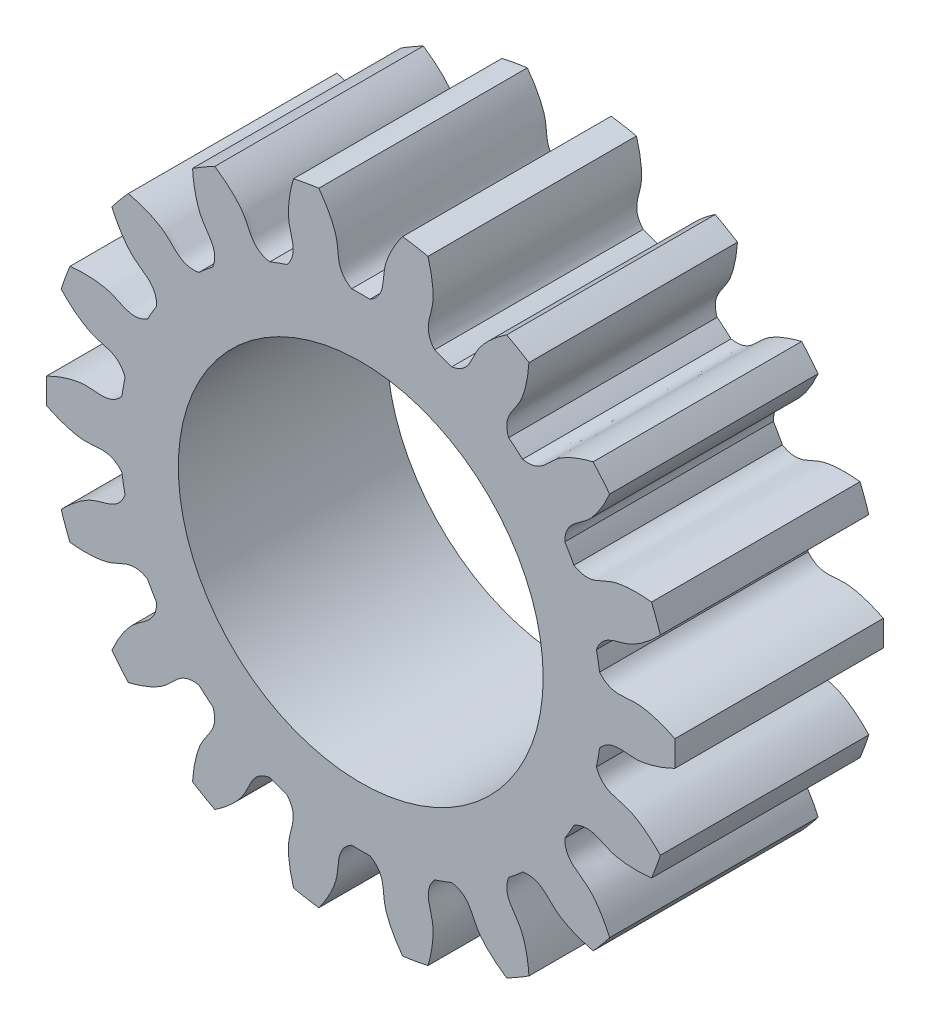
from build123d import *

# Parameters (mm, degrees)
SKETCH1_R           = 12.0625
BOSS_EXTRUDE1_DEPTH = 8
CUT_EXTRUDE1_DEPTH  = 19.841651002
CIRPATTERN1_COUNT   = 18
SKETCH4_R           = 7
CUT_EXTRUDE2_DEPTH  = 10


with BuildPart() as part:
    # Sketch1 → Boss-Extrude1 (new body)
    with BuildSketch(Plane.XY):
        Circle(SKETCH1_R)
    extrude(amount=BOSS_EXTRUDE1_DEPTH)

    # Sketch2 → Cut-Extrude1 (cut, through all)
    with BuildSketch(Plane.XY):
        with BuildLine():
            ThreePointArc((0.34899741, 9.243413915), (0, 9.25), (-0.34899741, 9.243413915))
            add(Edge.make_bspline(
                [(-0.34899741, 9.243413915), (-0.967596984, 9.594740668), (-0.816773651, 10.155382186), (-0.940364302, 10.666039056), (-0.94950446, 10.700802309), (-0.960495637, 10.739443489), (-0.97349239, 10.781901469), (-0.988652454, 10.828109672), (-1.006130135, 10.877997009), (-1.026078201, 10.93148765), (-1.048647143, 10.988501161), (-1.07398523, 11.048952534), (-1.102238338, 11.112752257), (-1.133549844, 11.179806369), (-1.168060499, 11.25001653), (-1.205908315, 11.323280084), (-1.247228447, 11.399490134), (-1.29215308, 11.478535614), (-1.340811315, 11.560301366), (-1.393329059, 11.64466822), (-1.44982892, 11.731513073), (-1.510430095, 11.820708981), (-1.575248268, 11.912125239), (-1.644395509, 12.005627475), (-1.717980173, 12.101077743), (-1.7961068, 12.198334618), (-1.878876025, 12.297253295), (-1.966384478, 12.397685684), (-2.058724701, 12.499480521), (-2.155985053, 12.602483466), (-2.258249629, 12.706537214), (-2.365598176, 12.811481602), (-2.478106012, 12.917153723), (-2.59584395, 13.023388036), (-2.71887822, 13.130016487), (-2.84727041, 13.23686862), (-2.981077352, 13.343771702), (-3.169013167, 13.487859202), (-3.314918218, 13.592849249), (-3.414675506, 13.661716548)],
                knots=[0, 0, 0, 0, 0.27435327, 0.280121527, 0.286658885, 0.293965344, 0.302040904, 0.310885565, 0.320499326, 0.330882189, 0.342034153, 0.353955217, 0.366645382, 0.380104649, 0.394333016, 0.409330484, 0.425097053, 0.441632723, 0.458937494, 0.477011366, 0.495854339, 0.515466413, 0.535847588, 0.556997863, 0.57891724, 0.601605717, 0.625063296, 0.649289975, 0.674285755, 0.700050637, 0.726584619, 0.753887702, 0.781959886, 0.810801171, 0.840411557, 0.870791044, 0.901939631, 0.93385732, 1, 1, 1, 1], degree=3))
            ThreePointArc((-3.414675506, 13.661716548), (0, 14.081992325), (3.414675506, 13.661716548))
            add(Edge.make_bspline(
                [(0.34899741, 9.243413915), (0.967596984, 9.594740668), (0.816773651, 10.155382186), (0.940364302, 10.666039056), (0.94950446, 10.700802309), (0.960495637, 10.739443489), (0.97349239, 10.781901469), (0.988652454, 10.828109672), (1.006130135, 10.877997009), (1.026078201, 10.93148765), (1.048647143, 10.988501161), (1.07398523, 11.048952534), (1.102238338, 11.112752257), (1.133549844, 11.179806369), (1.168060499, 11.25001653), (1.205908315, 11.323280084), (1.247228447, 11.399490134), (1.29215308, 11.478535614), (1.340811315, 11.560301366), (1.393329059, 11.64466822), (1.44982892, 11.731513073), (1.510430095, 11.820708981), (1.575248268, 11.912125239), (1.644395509, 12.005627475), (1.717980173, 12.101077743), (1.7961068, 12.198334618), (1.878876025, 12.297253295), (1.966384478, 12.397685684), (2.058724701, 12.499480521), (2.155985053, 12.602483466), (2.258249629, 12.706537214), (2.365598176, 12.811481602), (2.478106012, 12.917153723), (2.59584395, 13.023388036), (2.71887822, 13.130016487), (2.84727041, 13.23686862), (2.981077352, 13.343771702), (3.169013167, 13.487859202), (3.314918218, 13.592849249), (3.414675506, 13.661716548)],
                knots=[0, 0, 0, 0, 0.27435327, 0.280121527, 0.286658885, 0.293965344, 0.302040904, 0.310885565, 0.320499326, 0.330882189, 0.342034153, 0.353955217, 0.366645382, 0.380104649, 0.394333016, 0.409330484, 0.425097053, 0.441632723, 0.458937494, 0.477011366, 0.495854339, 0.515466413, 0.535847588, 0.556997863, 0.57891724, 0.601605717, 0.625063296, 0.649289975, 0.674285755, 0.700050637, 0.726584619, 0.753887702, 0.781959886, 0.810801171, 0.840411557, 0.870791044, 0.901939631, 0.93385732, 1, 1, 1, 1], degree=3))
        make_face()
    cut_extrude1 = extrude(amount=CUT_EXTRUDE1_DEPTH, mode=Mode.SUBTRACT)

    # CirPattern1: Cut-Extrude1 ×18 about axis
    cirpattern1_axis = Axis((0, 0, -0.4), (0, 0, 1))
    for i in range(1, CIRPATTERN1_COUNT):
        add(cut_extrude1.rotate(cirpattern1_axis, i * 360 / CIRPATTERN1_COUNT), mode=Mode.SUBTRACT)

    # Sketch4 → Cut-Extrude2 (cut)
    with BuildSketch(Plane.XY.offset(8)):
        Circle(SKETCH4_R)
    extrude(amount=-CUT_EXTRUDE2_DEPTH, mode=Mode.SUBTRACT)


solid = part.part
